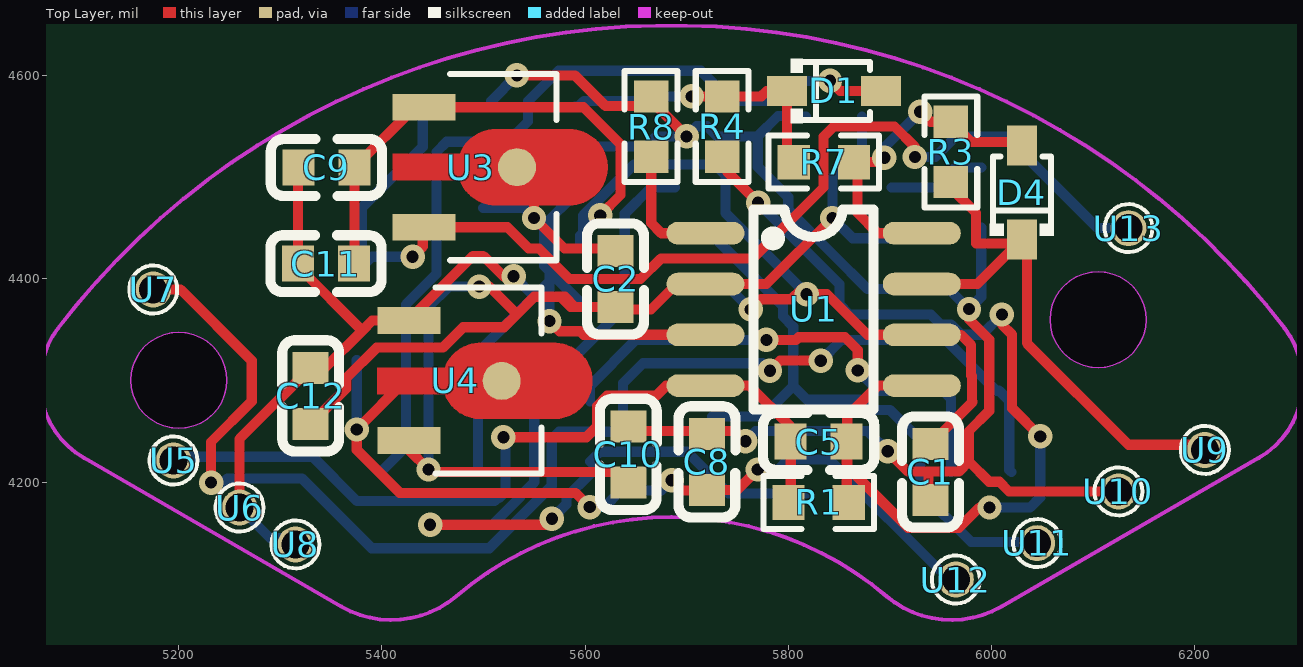
[diagram p0: Top Layer view]
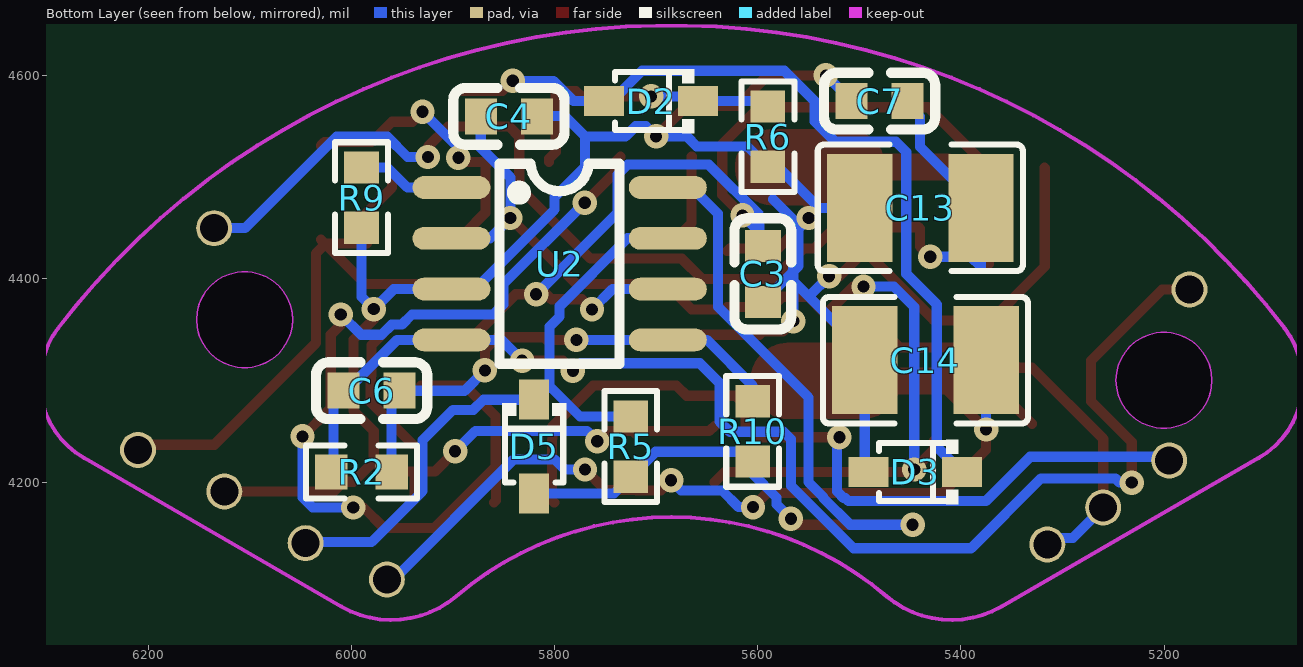
[diagram p1: Bottom Layer view, seen from below]
# Altium PCB MISC51764.pcbdoc
Units mil, origin at the board's own origin, x right, y up, seen from the top; angles counter-clockwise.
Board outline 5075 x 3290 mil, 2 copper layers (Top Layer, Bottom Layer), stack 2.757 mil thick; 42 components, 17 nets, 89 pads, 36 vias.

## Layer stack, top to bottom
Top Solder Mask Layer: solder mask 0.394, Dk 3.3
Top Layer: signal copper 1.379
Bottom Layer: signal copper 1.378
Bottom Solder Mask Layer: solder mask 0.394, Dk 3.3

## Board outline
7825,2750 2750,2750 2750,6040 7825,6040
cut-out: 6152.29,4359.89 cw(c6105.05,4359.89) 6057.8,4359.89 cw(c6105.05,4359.89)
cut-out: 5247.43,4300.23 cw(c5200.18,4300.23) 5152.94,4300.23 cw(c5200.18,4300.23)

## Design rules (kind name [scope] priority, off if disabled: settings)
BoardOutlineClearance Default_1 [All] p2: genericclearance=4 ignorepadtopadclearanceinfootprint=FALSE except(0: Arc-SplitContinuation Track-SplitContinuation SMDPad-SplitContinuation THPad-SplitContinuation Via-SplitContinuation Fill-SplitContinuation Region-SplitContinuation Poly-SplitContinuation Text-SplitContinuation Hole-SplitContinuation; 6: Arc-OutlineEdge Track-OutlineEdge SMDPad-OutlineEdge THPad-OutlineEdge Via-OutlineEdge Fill-OutlineEdge Region-OutlineEdge Poly-OutlineEdge Text-OutlineEdge Hole-OutlineEdge SMDPad-CutoutEdge THPad-CutoutEdge Via-CutoutEdge Fill-CutoutEdge Region-CutoutEdge Text-CutoutEdge; 6.9: Hole-CutoutEdge; 10: Poly-CutoutEdge; 11.8: Arc-CutoutEdge Track-CutoutEdge)
Clearance Default [All] p1: gap=4 ignorepadtopadclearanceinfootprint=FALSE except(6: SMDPad-Track SMDPad-SMDPad THPad-Track SMDPad-THPad THPad-THPad Track-Via SMDPad-Via THPad-Via Via-Via Fill-Track Region-Track Fill-SMDPad Region-SMDPad Fill-THPad Region-THPad Fill-Via Region-Via Fill-Fill Fill-Region Region-Region Arc-Track Arc-SMDPad Arc-THPad Arc-Via Fill-Arc Region-Arc Arc-Arc Text-Track SMDPad-Text Text-THPad Text-Via Fill-Text Region-Text Arc-Text Text-Text; 6.9: Hole-Track Hole-SMDPad Hole-THPad Hole-Via Fill-Hole Region-Hole Hole-Arc Hole-Text; 10: Poly-Track Poly-SMDPad Poly-THPad Poly-Via Poly-Fill Poly-Region Poly-Poly Poly-Arc Poly-Text Poly-Hole)
DiffPairsRouting differentialPair [All] p1: maxlimit=6 minlimit=5 mostfreqgap=6 toplayer_minwidth=5 toplayer_prefwidth=100 toplayer_maxwidth=100 toplayer_mingap=5 toplayer_prefgap=6 toplayer_maxgap=6 bottomlayer_minwidth=5 bottomlayer_prefwidth=100 bottomlayer_maxwidth=100 bottomlayer_mingap=5 bottomlayer_prefgap=6 bottomlayer_maxgap=6 maxuncoupledlength=10
HoleToHoleClearance otherClearance [All] p1: gap=11.8 allowstackedmicrovias=TRUE
Length netLength [All] p1: minlimit=0 maxlimit=0
MatchedLengths netLengthTolerance [All] p1: tolerance=1000
PasteMaskExpansion pasteMaskExpansion [All] p1: expansion=0
PlaneConnect innerPlane [All] p1: planeconnectstyle=Relief reliefexpansion=20 reliefentries=4 reliefconductorwidth=10 reliefairgap=10
PolygonConnect copperRegion [All] p1: connectstyle=Relief reliefconductorwidth=10 reliefentries=4 polygonreliefangle="90 Angle" airgapwidth=10 via.connectstyle=Relief via.reliefconductorwidth=10 via.reliefentries=4 via.polygonreliefangle="90 Angle" via.airgapwidth=10
RoutingVias Default_3 [All] p1: holewidth=12 width=24 viastyle="Through Hole" minholewidth=12 minwidth=24 maxholewidth=1181 maxwidth=1969
SolderMaskExpansion Common [IsVia] p1: expansion=-1000 istentingtop=TRUE
SolderMaskExpansion Common [All] p2: expansion=2 istentingtop=FALSE
Width Default_2 [All] p1: maxlimit=1000 minlimit=10 preferedwidth=10

## Components (designator, comment, footprint, x,y, rotation, side; value= is the part's Value field where it differs from the comment)
C1 "47nF" C0603 5940,4210 r90 top
C2 "47nF" C0603 5630,4400 r270 top
C3 "47nF" C0603 5595,4405 r90 bottom
C4 "47nF" C0603 5845,4560 r0 bottom
C5 "33pF" C0603 5830,4240 r0 top
C6 "33pF" C0603 5980,4290 r180 bottom
C7 "100nF" C0603 5480,4575 r180 bottom
C8 "100nF" C0603 5720,4220 r270 top
C9 "330nF" C0603 5345.43,4509.7 r0 top
C10 "330nF" C0603 5642.56,4227.44 r270 top
C11 "1uF" C0603 5345,4415 r0 top
C12 "1uF" C0603 5330,4285 r270 top
C13 "22uF" C1210 5440,4470 r0 bottom
C14 "22uF" C1210 5435,4320 r0 bottom
D1 "1N4148WS-7-F" SOD-323_L1.8-W1.3-LS2.5-RD 5845,4585 r0 top
D2 "1N4148WS-7-F" SOD-323_L1.8-W1.3-LS2.5-RD 5705,4575 r0 bottom
D3 "1N4148WS-7-F" SOD-323_L1.8-W1.3-LS2.5-RD 5445,4210 r0 bottom
D4 "1N4148WS-7-F" SOD-323_L1.8-W1.3-LS2.5-RD 6030,4485 r90 top
D5 "1N4148WS-7-F" SOD-323_L1.8-W1.3-LS2.5-RD 5820,4235 r270 bottom
R1 "1.5M" R0603 5830,4180 r0 top
R2 "1.5M" R0603 5990,4210 r180 bottom
R3 "205K" R0603 5960,4525 r270 top
R4 "4.7K" R0603 5735,4550 r90 top
R5 "200K" R0603 5725,4235 r90 bottom
R6 "20K" R0603 5590,4540 r90 bottom
R7 "33K" R0603 5835,4515 r0 top
R8 "33R" R0603 5665,4550 r90 top
R9 "33R" R0603 5990,4480 r270 bottom
R10 "11K" R0603 5605,4250 r270 bottom
U1 "LT1057IS8#PBF" SOIC-8_L5.0-W4.0-P1.27-LS6.0-BL 5825,4370 r270 top
U2 "LT1057IS8#PBF" SOIC-8_L5.0-W4.0-P1.27-LS6.0-BL 5795,4415 r270 bottom
U3 "L78L12ABUTR" SOT-89-3_L4.5-W2.5-P1.50-LS4.2-BR 5495,4510 r180 top
U4 "L79L12ACUTR" SOT-89-3_L4.5-W2.5-P1.50-LS4.2-TL 5480,4300 r0 top
U5 "MTBD1-D011000" CR100 5195,4221.29 r0 top
U6 "MTBD1-D011000" CR100 5260,4175 r0 top
U7 "MTBD1-D011000" CR100 5175,4389.57 r0 top
U8 "MTBD1-D011000" CR100 5315,4138.71 r0 top
U9 "MTBD1-D011000" CR100 6210,4231.72 r0 top
U10 "MTBD1-D011000" CR100 6125,4190.86 r0 top
U11 "MTBD1-D011000" CR100 6045,4140 r0 top
U12 "MTBD1-D011000" CR100 5965,4104.14 r0 top
U13 "MTBD1-D011000" CR100 6135,4450 r0 top

## Footprints (in the part's own frame and the unit in brackets; to place one, negate y for a bottom-side part, rotate by r counter-clockwise, add the part's x,y. Pads: shape width x height; smd on the part's side, far side on the other; paste and mask are expansions set on the pad)
C0603 [mm]
  rect 0.8x0.9 smd paste+0 mask+0.051: 1(-0.7,0) 2(0.7,0)
  silkscreen extent -1.39,-0.71 1.39,0.71
C1210 [mm]
  rect 1.635x2.7 smd paste-100 mask+0.051: 1(-1.517,0) 2(1.517,0)
  silkscreen extent -2.56,-1.58 2.56,1.58
CR100 [mm]
  round 0.9 hole 0.7 paste+0 mask+0.05: 1(0,0)
  silkscreen extent -0.6,-0.6 0.6,0.6
R0603 [mil]
  rect 31.75x34.02 smd paste-3937.01 mask+2: 1(-29.65,0) 2(29.65,0)
  silkscreen extent -55,-26 55,26
SOD-323_L1.8-W1.3-LS2.5-RD [mm]
  rect 1x0.75 smd paste+0 mask+0.051: 1(-1.173,0) 2(1.173,0)
  silkscreen extent -1.08,-0.8 0.9,0.8
SOIC-8_L5.0-W4.0-P1.27-LS6.0-BL [mil]
  oval 22.38x76.78 smd paste+0 mask+2: 1(-75,-106.5) 2(-25,-106.5) 3(25,-106.5) 4(75,-106.5) 5(75,106.5) 6(25,106.5) 7(-25,106.5) 8(-75,106.5)
  silkscreen extent -98,-59 98,59
SOT-89-3_L4.5-W2.5-P1.50-LS4.2-BR [mm]
  rect 1.575x0.672 smd paste+0 mask+0.051: 1(1.356,-1.5) 3(1.356,1.5)
  round 0.95 smd: 2(-0.966,0)
  Top Layer region: -2.283,0.95 -0.429,0.95 -0.384,0.949 -0.34,0.946 -0.296,0.94 -0.252,0.933 -0.208,0.924 -0.165,0.912 -0.123,0.899 -0.081,0.884 -0.04,0.866 0,0.847 0.04,0.826 0.078,0.803 0.115,0.779 0.151,0.752 0.185,0.724 0.219,0.695 0.251,0.664 0.281,0.631 0.31,0.597 0.337,0.562 0.362,0.525 0.386,0.488 0.408,0.449 0.428,0.409 0.447,0.33 2.144,0.33 2.144,-0.33 0.447,-0.33 0.428,-0.409 0.408,-0.449 0.386,-0.488 0.362,-0.526 0.337,-0.562 0.31,-0.597 0.281,-0.631 0.251,-0.664 0.219,-0.695 0.185,-0.725 0.151,-0.753 0.115,-0.779 0.078,-0.804 0.04,-0.827 0,-0.848 -0.04,-0.867 -0.081,-0.884 -0.123,-0.899 -0.165,-0.913 -0.208,-0.924 -0.252,-0.934 -0.296,-0.941 -0.34,-0.946 -0.384,-0.949 -0.429,-0.95 -2.283,-0.95 -2.328,-0.949 -2.372,-0.946 -2.416,-0.941 -2.46,-0.934 -2.504,-0.924 -2.547,-0.913 -2.589,-0.899 -2.631,-0.884 -2.672,-0.867 -2.713,-0.848 -2.752,-0.827 -2.79,-0.804 -2.827,-0.779 -2.863,-0.753 -2.898,-0.725 -2.931,-0.695 -2.963,-0.664 -2.993,-0.631 -3.022,-0.597 -3.049,-0.562 -3.075,-0.526 -3.098,-0.488 -3.12,-0.449 -3.141,-0.409 -3.159,-0.369 -3.175,-0.327 -3.189,-0.285 -3.202,-0.242 -3.212,-0.199 -3.22,-0.155 -3.227,-0.111 -3.231,-0.067 -3.233,-0.022 -3.233,0.022 -3.231,0.067 -3.227,0.111 -3.22,0.155 -3.212,0.199 -3.202,0.242 -3.189,0.285 -3.175,0.327 -3.159,0.369 -3.141,0.409 -3.12,0.449 -3.098,0.488 -3.075,0.525 -3.049,0.562 -3.022,0.597 -2.993,0.631 -2.963,0.664 -2.931,0.695 -2.898,0.724 -2.863,0.752 -2.827,0.779 -2.79,0.803 -2.752,0.826 -2.713,0.847 -2.672,0.866 -2.631,0.884 -2.589,0.899 -2.547,0.912 -2.504,0.924 -2.46,0.933 -2.416,0.94 -2.372,0.946 -2.328,0.949
  silkscreen extent -1.95,-2.33 0.7,2.33
SOT-89-3_L4.5-W2.5-P1.50-LS4.2-TL [mm]
  rect 1.575x0.672 smd paste+0 mask+0.051: 1(-1.356,1.5) 3(-1.356,-1.5)
  round 0.95 smd: 2(0.966,-0.009)
  Top Layer region: 2.283,-0.959 0.429,-0.959 0.384,-0.958 0.34,-0.954 0.296,-0.949 0.252,-0.942 0.208,-0.933 0.165,-0.921 0.123,-0.908 0.081,-0.893 0.04,-0.875 0,-0.856 -0.04,-0.835 -0.078,-0.812 -0.115,-0.787 -0.151,-0.761 -0.185,-0.733 -0.219,-0.704 -0.251,-0.672 -0.281,-0.64 -0.31,-0.606 -0.337,-0.571 -0.362,-0.534 -0.386,-0.496 -0.408,-0.458 -0.428,-0.418 -0.447,-0.339 -2.144,-0.339 -2.144,0.321 -0.447,0.321 -0.428,0.401 -0.408,0.44 -0.386,0.479 -0.362,0.517 -0.337,0.553 -0.31,0.589 -0.281,0.623 -0.251,0.655 -0.219,0.686 -0.185,0.716 -0.151,0.744 -0.115,0.77 -0.078,0.795 -0.04,0.818 0,0.839 0.04,0.858 0.081,0.875 0.123,0.891 0.165,0.904 0.208,0.915 0.252,0.925 0.296,0.932 0.34,0.937 0.384,0.94 0.429,0.941 2.283,0.941 2.328,0.94 2.372,0.937 2.416,0.932 2.46,0.925 2.504,0.915 2.547,0.904 2.589,0.891 2.631,0.875 2.672,0.858 2.712,0.839 2.752,0.818 2.79,0.795 2.827,0.77 2.863,0.744 2.898,0.716 2.931,0.686 2.963,0.655 2.993,0.623 3.022,0.589 3.049,0.553 3.075,0.517 3.098,0.479 3.12,0.44 3.14,0.401 3.159,0.36 3.175,0.319 3.189,0.277 3.202,0.234 3.212,0.19 3.22,0.147 3.227,0.103 3.231,0.058 3.233,0.014 3.233,-0.031 3.231,-0.075 3.227,-0.12 3.22,-0.164 3.212,-0.208 3.202,-0.251 3.189,-0.294 3.175,-0.336 3.159,-0.377 3.14,-0.418 3.12,-0.458 3.098,-0.496 3.075,-0.534 3.049,-0.571 3.022,-0.606 2.993,-0.64 2.963,-0.672 2.931,-0.704 2.898,-0.733 2.863,-0.761 2.827,-0.787 2.79,-0.812 2.752,-0.835 2.712,-0.856 2.672,-0.875 2.631,-0.893 2.589,-0.908 2.547,-0.921 2.504,-0.933 2.46,-0.942 2.416,-0.949 2.372,-0.954 2.328,-0.958
  silkscreen extent -0.69,-2.33 1.96,2.33

## Via types
v1: diameter 24.02, hole 12, Top Layer to Bottom Layer, 36 vias

## Nets (pads, with @x,y where several pads share a name; then routed paths per layer and width w, separated by ;. In a path a pad name is that pad's centre, name@x,y a point inside that pad or via, vN(x,y) a via of type N, cw(c..) or ccw(c..) an arc to the next point about the centre after c; other vN are vias at no path point)
+12V: C1.2 C3.2 C9.2 C11.2 U1.6 U2.6 U3.1 | length 1267.4
  Top Layer w10: C11.2 5372.99,4419.7 C9.2 5432.34,4569.06 5441.61,4569.06 5598.51,4569.06 5635,4532.56 5635,4482.56 v1(5615,4462.56) ; v1(5763.11,4370) 5773.11,4380 5803.11,4380 5813.11,4390 v1(5818.11,4385) 5838.11,4385 5878.11,4345 U1.6 ; C1.2 5981.5,4279.06 5980.89,4279.67 5980.89,4304.19 5980,4305.08 5980,4335 5970,4345
  Bottom Layer w10: v1(5615,4462.56) C3.2@5598.11,4445.67 ; U2.6 5743.11,4390 v1(5763.11,4370) ; v1(5818.11,4385) 5738.11,4465 5738.11,4502.56 5728.11,4512.56 5648.11,4512.56 5598.11,4462.56 C3.2@5598.11,4445.67 ; C3.2@5598.11,4445.67 5598.11,4435.67 C3.2 5595,4442.56 C3.2@5598.11,4445.67
+15V: C7.2 C13.1 U3.3 U13.1 | length 1150.7
  Top Layer w10: v1(5430.26,4421.85) 5440.26,4431.85 5440.26,4449.6 U3.3 5523.71,4450.95 5544.66,4430 5554.66,4430 5584.66,4400 5654.66,4400 5674.66,4420 5764.66,4420 5834.66,4490 5834.66,4540 5844.66,4550 5904.66,4550 5924.66,4530 v1(5924.66,4520)
  Bottom Layer w10: v1(5430.26,4421.85) 5390.26,4421.85 5380.26,4411.85 C13.1 5440.26,4530 5440.26,4560 5452.44,4572.18 C7.2 ; v1(5924.66,4520) 5944.66,4520 5964.66,4540 6014.66,4540 6104.66,4450 U13.1
-12V: C2.2 C4.2 C10.2 C12.2 U1.2 U2.2 U4.3 | length 1314.9
  Top Layer w10: C12.2 5365,4292.44 5365,4302.44 5395,4332.44 5460,4332.44 5480,4352.44 5520,4352.44 5532.97,4365.41 ; U4.3@5426.61,4240.95 5426.61,4231.78 v1(5445.94,4212.44) 5448.5,4209.88 5632.56,4209.88 C10.2 ; v1(5495.94,4392.44) 5505.94,4392.44 5532.97,4365.41 ; v1(5843.5,4460) 5778.5,4395 U1.2 5690,4395 5665,4370 5632.45,4370 C2.2 5590,4372.44 ; 5532.97,4365.41 5550,4382.44 5575.94,4382.44 ; 5575.94,4382.44 5585.94,4372.44 5590,4372.44 ; 5575.94,4382.44 5580,4382.44 5590,4372.44
  Bottom Layer w10: v1(5445.94,4212.44) 5445.94,4372.44 5465.94,4392.44 v1(5495.94,4392.44) ; C4.2 5872.56,4529.06 5843.5,4500 v1(5843.5,4460) 5863.5,4440 U2.2
-15V: C8.2 C14.1 U4.2 U12.1 | length 956
  Top Layer w10: U4.2@5533.4,4299.67 5423.08,4299.67 v1(5375.26,4251.85) 5375.26,4231.85 5417.68,4189.44 5590.61,4189.44 v1(5604.63,4175.42) ; v1(5685.26,4201.85) 5695.26,4191.85 5719.41,4191.85 C8.2 5750,4192.44 v1(5770,4212.44)
  Bottom Layer w10: v1(5375.26,4251.85) C14.1 ; v1(5604.63,4175.42) 5618.82,4175.42 5635.26,4191.85 5675.26,4191.85 v1(5685.26,4201.85) ; v1(5770,4212.44) 5790,4212.44 5800,4222.44 5840,4222.44 5958.3,4104.14 U12.1
A_IN+1: R8.1 U1.1 | length 122.9
  Top Layer w10: R8.1 5665.11,4515 5665.11,4455 5675.11,4445 U1.1
A_IN+2: C1.1 C2.1 C3.1 C4.1 C7.1 C8.1 C9.1 C10.1 C11.1 C12.1 C13.2 C14.2 D3.2 R6.1 R8.2 R9.2 U1.3 U2.3 U3.2 U4.1 U6.1 U8.1 U10.1 | length 3191.8
  Top Layer w10: U6.1 5260,4242.56 C12.1 5344.11,4312.56 5380.6,4349.06 ; C9.1 5317.44,4509.27 C11.1 5317.44,4412.22 5380.6,4349.06 ; v1(5529.74,4402.7) 5519.74,4402.7 5499.74,4422.7 5489.74,4422.7 5429.74,4362.7 U4.1 5390.6,4359.06 5380.6,4349.06 ; v1(5532.9,4600.34) 5590,4600.34 5620,4570.34 R8.2@5670,4570.34 ; U3.2@5548.4,4510.01 5549.74,4508.66 v1(5549.74,4460) 5579.74,4430 5627.56,4430 C2.1 ; v1(5565,4358.5) 5575,4348.5 5595,4348.5 5598.5,4345 U1.3 ; C10.1 5647.9,4250.34 C8.1@5717.9,4250.34 ; R8.2 5665,4575.34 R8.2@5670,4570.34 ; v1(5700,4540.34) R8.2@5670,4570.34 ; C8.1 5720,4248.24 C8.1@5717.9,4250.34 ; v1(5757.9,4240.34) 5747.9,4250.34 C8.1@5717.9,4250.34 ; v1(5897.9,4230.34) 5917.9,4210.34 5937.9,4210.34 ; C1.1 5937.9,4184.54 5937.9,4210.34 ; v1(5977.9,4370.34) 5977.9,4360.34 5997.9,4340.34 5997.9,4270.34 5977.9,4250.34 5977.9,4220.34 ; U10.1 6017.38,4190.86 6007.9,4200.34 5997.9,4200.34 5977.9,4220.34 ; 5937.9,4210.34 5967.9,4210.34 5977.9,4220.34
  Bottom Layer w10: U6.1 5290,4145 5308.71,4145 U8.1 ; D3.2 5494.74,4213.57 C14.2 5499.74,4325 5499.74,4332.7 5549.74,4382.7 ; C13.2 5539.74,4470 ; C7.1 v1(5532.9,4600.34) ; v1(5529.74,4402.7) 5549.74,4382.7 ; v1(5565,4358.5) 5565,4397.96 ; 5565,4457.44 5565,4407.44 ; 5565,4458.5 5585,4478.5 ; C3.1 5569.74,4402.7 ; v1(5757.9,4240.34) 5767.9,4250.34 5877.9,4250.34 v1(5897.9,4230.34) ; C4.1 5810,4560.34 5790,4560.34 5770,4540.34 ; R9.2 5990,4382.44 v1(5977.9,4370.34) 5958.24,4390 U2.3 5878.24,4390 5843.63,4424.61 5800,4468.24 5800,4480.34 5770,4510.34 5770,4540.34 ; 5539.74,4470 v1(5549.74,4460) 5559.74,4450 5559.74,4412.7 5565,4407.44 ; 5539.74,4470 5579.74,4510 R6.1 5610,4530.34 5660,4530.34 5670,4540.34 v1(5700,4540.34) 5710,4550.34 5720,4550.34 5730,4540.34 5770,4540.34 ; 5549.74,4382.7 5565,4397.96 ; 5565,4397.96 5569.74,4402.7 ; 5565,4397.96 5565,4407.44 ; 5565,4407.44 5569.74,4402.7
A_IN-1: D4.2 R3.1 R7.2 U1.8 | length 328.7
  Top Layer w10: v1(5894.66,4519.32) 5890.34,4515 R7.2 5868.11,4511.55 5868.11,4465 5888.11,4445 U1.8 ; v1(5930,4564.66) 5940,4554.66 R3.1 5980,4534.66 6026.5,4534.66 D4.2
  Bottom Layer w10: v1(5894.66,4519.32) 5894.66,4529.32 v1(5930,4564.66)
A_IN-2: C5.1 R1.1 U1.4 U5.1 | length 812.3
  Top Layer w10: v1(5519.64,4244.26) 5601.14,4244.26 5611.89,4255 5611.89,4275 5621.89,4285 5670,4285 5680,4295 U1.4 5761.89,4295 5801.89,4255 5801.89,4245 C5.1 5802.44,4182.1 R1.1
  Bottom Layer w10: U5.1 5198.18,4221.29 5201.89,4225 5331.89,4225 5375.54,4181.36 5510.75,4181.36 5513.63,4184.24 5515.41,4184.24 5521.89,4190.72 5521.89,4242 v1(5519.64,4244.26)
A_OUT1: D4.1 R3.2 U1.7 U9.1 | length 547.4
  Top Layer w10: U1.7 5986.16,4395 D4.1@6025.53,4434.36 ; R3.2 5960,4489.89 5984.89,4465 5984.89,4435 D4.1@6024.89,4435 ; D4.1 D4.1@6025.53,4434.36 ; U9.1 6204.89,4236.83 6134.89,4236.83 6034.89,4336.83 6034.89,4425 D4.1@6025.53,4434.36
A_OUT2: C5.2 R1.2 R4.1 U1.5 | length 998.5
  Top Layer w10: R4.1 5740.34,4515 5740.34,4505 v1(5770.34,4475) ; R1.2 5857.56,4182.1 C5.2 C5.2@5858.11,4245 ; U1.5 5888.11,4295 5858.11,4265 C5.2@5858.11,4245 ; v1(5998.11,4175) 5988.11,4175 5968.11,4155 5918.11,4155 5858.11,4215 C5.2@5858.11,4245 ; v1(6010.34,4365) 6010.34,4355 6020.34,4345 6020.34,4272.77 v1(6048.11,4245)
  Bottom Layer w10: v1(5770.34,4475) 5850.34,4395 5850.34,4375 5860.34,4365 5940.34,4365 5950.34,4355 5960.34,4355 5970.34,4345 5990.34,4345 v1(6010.34,4365) ; v1(5998.11,4175) 6038.11,4175 6048.11,4185 v1(6048.11,4245)
B_IN+1: R9.1 U2.1 | length 96.6
  Bottom Layer w10: U2.1 5944.89,4490 5964.55,4509.66 R9.1
B_IN-1: D5.2 R5.1 R10.2 U2.8 | length 911.5
  Top Layer w10: v1(5447.57,4158.01) 5561.31,4158.01 v1(5567.37,4164.06)
  Bottom Layer w10: v1(5447.57,4158.01) 5508.98,4158.01 5535.89,4184.92 5535.89,4185.89 5550,4200 5550,4283.42 5639.11,4372.53 5639.11,4464.11 5665,4490 U2.8 ; v1(5567.37,4164.06) 5581.62,4178.31 5581.62,4184.95 R10.2@5605,4208.33 ; R10.2@5608.5,4210 5608.5,4216.84 R10.2 5614.66,4230 5700.34,4230 R5.1 5741.51,4188.84 D5.2
B_IN-2: C6.1 R2.1 U2.4 U7.1 | length 1314.1
  Top Layer w10: U7.1 5201.94,4389.57 5271.94,4319.57 5271.94,4279.57 5231.94,4239.57 v1(5231.94,4199.57) ; v1(5781.93,4309.57) 5791.93,4319.57 v1(5831.93,4319.57)
  Bottom Layer w10: v1(5231.94,4199.57) 5243.96,4199.57 5248.11,4203.72 5321.28,4203.72 5390,4135 5505.77,4135 5567.19,4196.42 5567.19,4242.19 5574.61,4249.61 5627.46,4249.61 5637.46,4259.61 5637.46,4297.46 5656.99,4316.99 5774.51,4316.99 v1(5781.93,4309.57) ; v1(5831.93,4319.57) 5852.37,4340 U2.4 5954.89,4340 6004.89,4290 C6.1 6017.56,4280 6017.56,4212.1 R2.1
B_OUT1: D5.1 R5.2 U2.7 U11.1 | length 642.6
  Bottom Layer w10: U2.7 5728.11,4440 5795,4373.11 5795,4363.11 5805,4353.11 5805,4294.66 ; R5.2 5775,4264.66 5805,4294.66 ; U11.1 6043.83,4141.17 5980,4141.17 5930,4191.17 5930,4241.17 5900,4271.17 5880,4271.17 5870,4281.17 D5.1 5818.5,4281.17 5805,4294.66
B_OUT2: C6.2 R2.2 R10.1 U2.5 | length 499.3
  Top Layer w10: v1(5778.5,4340) 5807.76,4340 5810.33,4342.58 5855.93,4342.58 5868.5,4330 v1(5868.5,4310)
  Bottom Layer w10: R10.1 5605,4295 5650,4340 U2.5 v1(5778.5,4340) ; v1(5868.5,4310) 5888.5,4290 C6.2 5960.34,4282.1 R2.2
D1_1: D1.1 D2.1 R4.2 R6.2 R7.1 | length 287.9
  Top Layer w10: v1(5705,4579.66) R4.2 5773.5,4579.66 5778.84,4585 D1.1 5798.84,4525 5805.34,4518.5 R7.1
  Bottom Layer w10: R6.2 5593.5,4569.66 5598.84,4575 D2.1 5660.34,4575 5665,4579.66 v1(5705,4579.66)
D1_2: D1.2 D2.2 D3.1 | length 864.8
  Top Layer w10: v1(5841.17,4595) 5851.17,4585 D1.2
  Bottom Layer w10: D3.1 5423.84,4235 5423.84,4375 5453.84,4405 5453.84,4525 5463.84,4535 5523.84,4535 5543.84,4555 5543.84,4575 5573.84,4605 5713.84,4605 5743.84,4575 5771.17,4575 ; D2.2 5781.17,4575 5801.17,4595 v1(5841.17,4595)

## Keep-outs
Board Outline Layer:
  region: 6152.29,4359.89 cw(c6105.05,4359.89) 6057.8,4359.89 cw(c6105.05,4359.89)
  circle w0.1: c6105.05,4359.89 r47.24
  region: 6152.29,4359.89 6151.92,4353.97 6150.81,4348.14 6148.97,4342.5 6146.45,4337.13 6143.27,4332.12 6139.49,4327.55 6135.16,4323.49 6130.36,4320 6125.16,4317.14 6119.64,4314.96 6113.9,4313.48 6108.01,4312.74 6102.08,4312.74 6096.19,4313.48 6090.45,4314.96 6084.93,4317.14 6079.73,4320 6074.93,4323.49 6070.61,4327.55 6066.82,4332.12 6063.65,4337.13 6061.12,4342.5 6059.29,4348.14 6058.17,4353.97 6057.8,4359.89 6058.17,4365.81 6059.29,4371.64 6061.12,4377.28 6063.65,4382.65 6066.82,4387.66 6070.61,4392.23 6074.93,4396.29 6079.73,4399.78 6084.93,4402.64 6090.45,4404.82 6096.19,4406.29 6102.08,4407.04 6108.01,4407.04 6113.9,4406.29 6119.64,4404.82 6125.16,4402.64 6130.36,4399.78 6135.16,4396.29 6139.49,4392.23 6143.27,4387.66 6146.45,4382.65 6148.97,4377.28 6150.81,4371.64 6151.92,4365.81
  region: 5247.43,4300.23 cw(c5200.18,4300.23) 5152.94,4300.23 cw(c5200.18,4300.23)
  circle w0.1: c5200.18,4300.23 r47.24
  region: 5247.43,4300.23 5247.05,4294.31 5245.94,4288.48 5244.11,4282.84 5241.58,4277.47 5238.4,4272.46 5234.62,4267.89 5230.3,4263.83 5225.5,4260.34 5220.3,4257.48 5214.78,4255.3 5209.03,4253.83 5203.15,4253.08 5197.22,4253.08 5191.33,4253.83 5185.58,4255.3 5180.07,4257.48 5174.87,4260.34 5170.07,4263.83 5165.74,4267.89 5161.96,4272.46 5158.78,4277.47 5156.26,4282.84 5154.42,4288.48 5153.31,4294.31 5152.94,4300.23 5153.31,4306.15 5154.42,4311.98 5156.26,4317.62 5158.78,4322.99 5161.96,4328 5165.74,4332.57 5170.07,4336.63 5174.87,4340.12 5180.07,4342.98 5185.58,4345.16 5191.33,4346.64 5197.22,4347.38 5203.15,4347.38 5209.03,4346.64 5214.78,4345.16 5220.3,4342.98 5225.5,4340.12 5230.3,4336.63 5234.62,4332.57 5238.4,4328 5241.58,4322.99 5244.11,4317.62 5245.94,4311.98 5247.05,4306.15
  lines w3.94: 5081.3,4351.42 cw(c5685,3890) 6288.7,4351.42 cw(c6219.88,4298.83) 6263.19,4223.82 6009.7,4077.46 cw(c5960.48,4162.7) 5896.71,4087.73 ccw(c5685,3838.82) 5473.29,4087.73 cw(c5409.52,4162.7) 5360.3,4077.46 5106.81,4223.82 cw(c5150.12,4298.83) 5081.3,4351.42

## Silkscreen, mask and mechanical layers (free items; w line width, h text height)
Mechanical Layer:
  circle w0.1: c6105.05,4359.89 r47.24
  circle w0.1: c5200.18,4300.23 r47.24